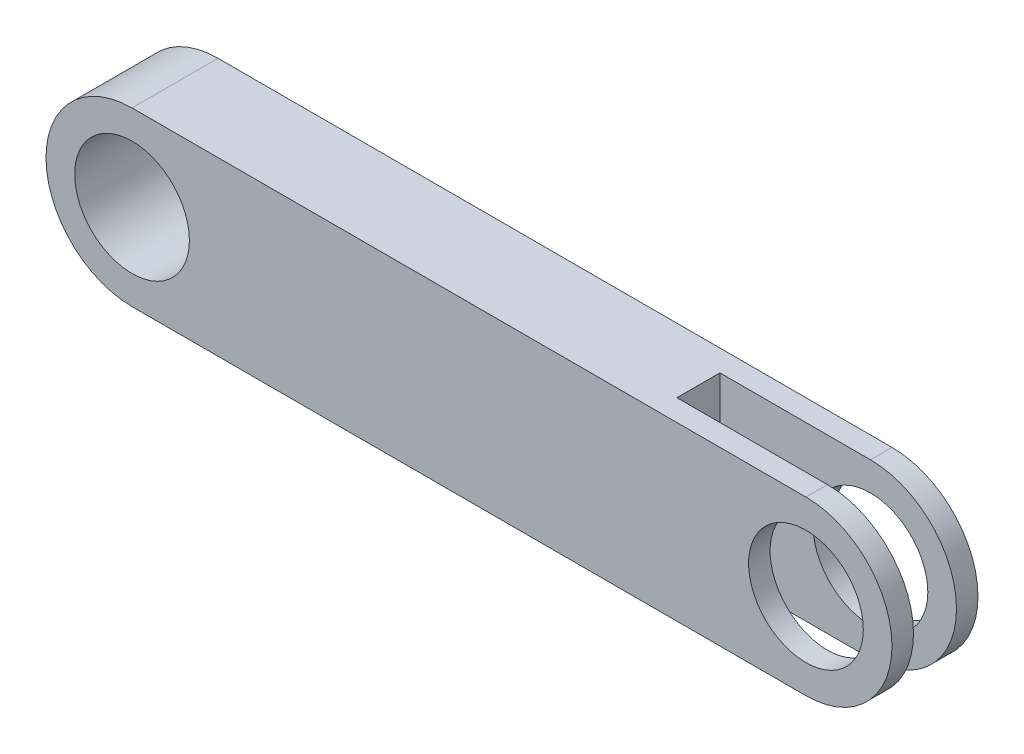
from build123d import *

# Parameters (mm, degrees)
BOSS_EXTRUDE1_DEPTH = 6
SKETCH2_W           = 33
SKETCH2_H           = 3
CUT_EXTRUDE1_DEPTH  = 35
SKETCH3_R           = 4
CUT_EXTRUDE2_DEPTH  = 35


with BuildPart() as part:
    # Sketch1 → Boss-Extrude1 (new body)
    with BuildSketch(Plane.XY):
        with BuildLine():
            Line((23.5, -6), (-23.5, -6))
            ThreePointArc((-23.5, -6), (-29.5, 0), (-23.5, 6))
            Line((-23.5, 6), (23.5, 6))
            ThreePointArc((23.5, 6), (29.5, 0), (23.5, -6))
        make_face()
    extrude(amount=BOSS_EXTRUDE1_DEPTH)

    # Sketch2 → Cut-Extrude1 (cut)
    with BuildSketch(Plane(origin=(0, 6, 0), x_dir=(1, 0, 0), z_dir=(0, 1, 0))):
        with Locations((29.5, -3)):
            Rectangle(SKETCH2_W, SKETCH2_H)
    extrude(amount=-CUT_EXTRUDE1_DEPTH, mode=Mode.SUBTRACT)

    # Sketch3 → Cut-Extrude2 (cut)
    with BuildSketch(Plane.XY.offset(6)):
        with Locations((23.5, 0)):
            Circle(SKETCH3_R)
        with Locations((-23.5, 0)):
            Circle(SKETCH3_R)
    extrude(amount=-CUT_EXTRUDE2_DEPTH, mode=Mode.SUBTRACT)


solid = part.part
